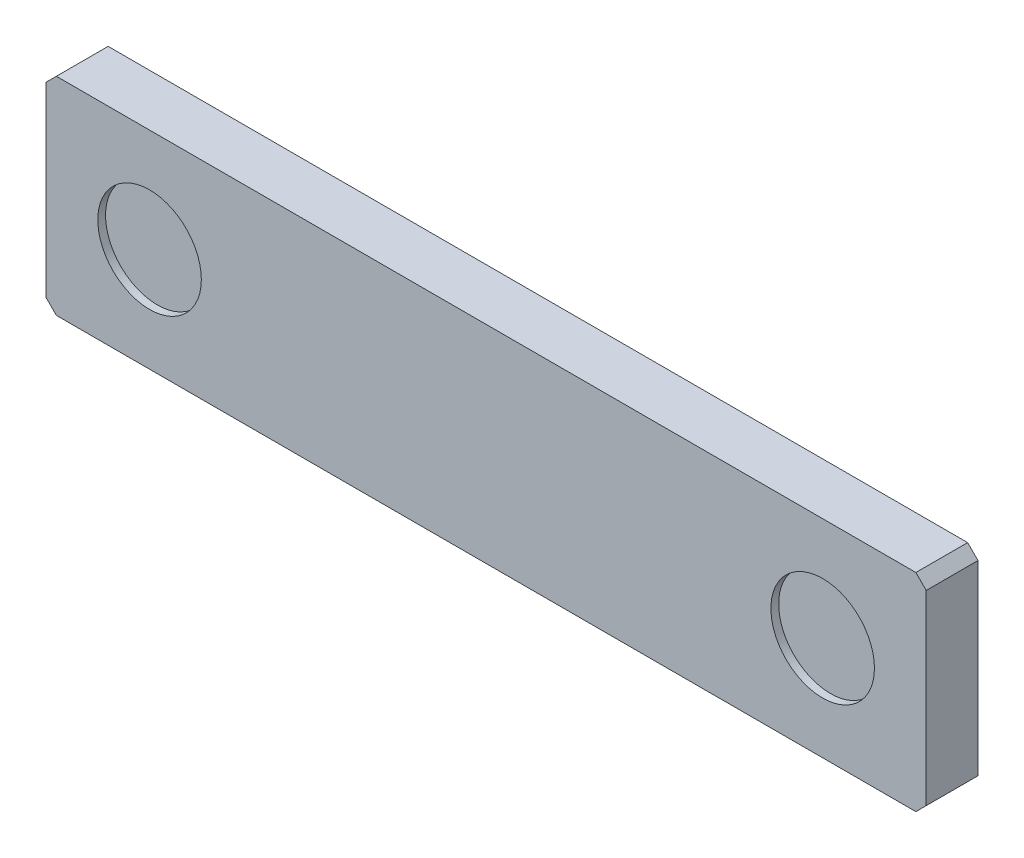
from build123d import *

# Parameters (mm, degrees)
SKETCH_1_W          = 170
SKETCH_1_H          = 40
EXTRUDE_1_DEPTH     = 10
SKETCH_2_R          = 10
CUT_EXTRUDE_1_DEPTH = 1.5
CHAMFER_1_SIZE      = 2


with BuildPart() as part:
    # 草图1 → 凸台-拉伸1 (new body)
    with BuildSketch(Plane.XY):
        Rectangle(SKETCH_1_W, SKETCH_1_H)
    extrude(amount=EXTRUDE_1_DEPTH)

    # 草图2 → 切除-拉伸1 (cut)
    with BuildSketch(Plane.XY.offset(10)):
        with Locations((-65, 0)):
            Circle(SKETCH_2_R)
        with Locations((65, 0)):
            Circle(SKETCH_2_R)
    extrude(amount=-CUT_EXTRUDE_1_DEPTH, mode=Mode.SUBTRACT)

    # 倒角1
    chamfer_1_edges = [part.edges().sort_by_distance(p)[0] for p in [
        (85, -20, 5),
        (-85, -20, 5),
        (-85, 20, 5),
        (85, 20, 5),
    ]]
    chamfer(chamfer_1_edges, length=CHAMFER_1_SIZE)


solid = part.part
